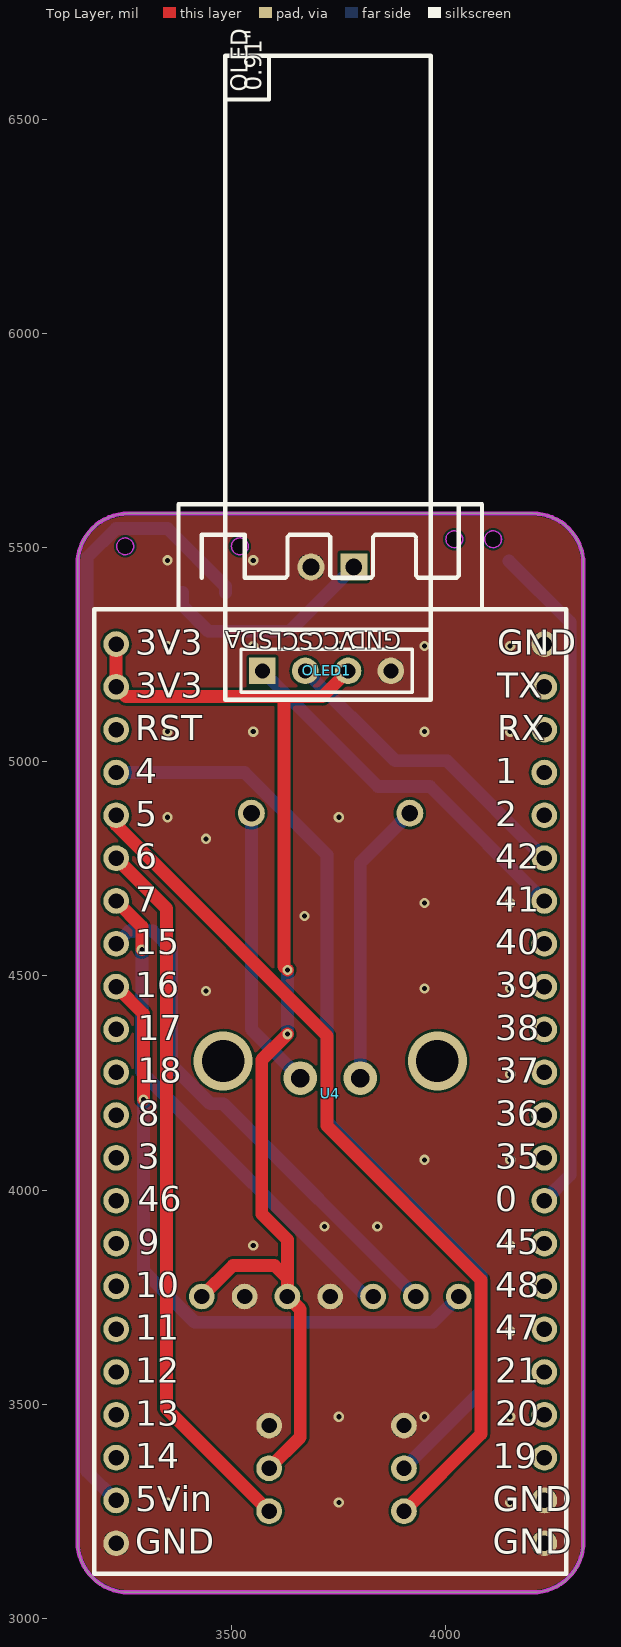
[diagram p0: Top Layer view]
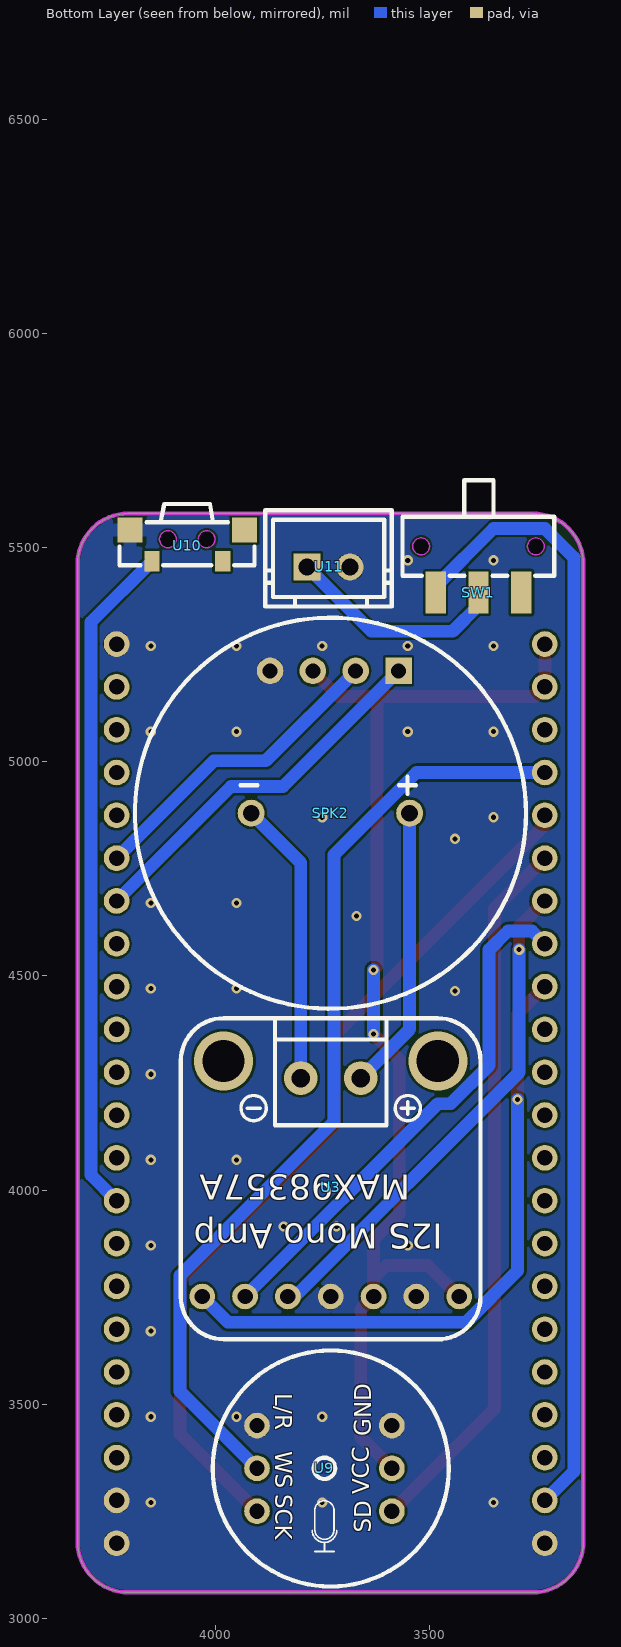
[diagram p1: Bottom Layer view, seen from below]
# Altium PCB MISC49945.pcbdoc
Units mil, origin at the board's own origin, x right, y up, seen from the top; angles counter-clockwise.
Board outline 1181.1 x 2519.68 mil, 2 copper layers (Top Layer, Bottom Layer), stack 62.206 mil thick; 8 components, 43 nets, 74 pads, 40 vias.

## Layer stack, top to bottom
Top Solder Mask Layer: solder mask 0.394, Dk 3.3
Top Layer: signal copper 1.379
Dielectric1: surface 59.449, FR4, Dk 4.5
Bottom Layer: signal copper 1.378
Bottom Solder Mask Layer: solder mask 0.394, Dk 3.3

## Board outline
3258.11,5580 ccw(c3258.11,5461.89) 3140,5461.89 3140,3178.43 ccw(c3258.11,3178.43) 3258.11,3060.32 4202.99,3060.32 ccw(c4202.99,3178.43) 4321.1,3178.43 4321.1,5461.89 ccw(c4202.99,5461.89) 4202.99,5580

## Design rules (kind name [scope] priority, off if disabled: settings)
BoardOutlineClearance Plane_Default_1 [All] p2 off: genericclearance=6 ignorepadtopadclearanceinfootprint=FALSE except(0: Arc-SplitContinuation Track-SplitContinuation SMDPad-SplitContinuation THPad-SplitContinuation Via-SplitContinuation Fill-SplitContinuation Region-SplitContinuation Poly-SplitContinuation Text-SplitContinuation Hole-SplitContinuation; 6: Arc-OutlineEdge Track-OutlineEdge SMDPad-OutlineEdge THPad-OutlineEdge Via-OutlineEdge Fill-OutlineEdge Region-OutlineEdge Poly-OutlineEdge Text-OutlineEdge Hole-OutlineEdge Arc-CutoutEdge Track-CutoutEdge SMDPad-CutoutEdge THPad-CutoutEdge Via-CutoutEdge Fill-CutoutEdge Region-CutoutEdge Poly-CutoutEdge Text-CutoutEdge Hole-CutoutEdge)
BoardOutlineClearance Copper_Default_1 [All] p4 off: genericclearance=6 ignorepadtopadclearanceinfootprint=FALSE except(0: Arc-SplitContinuation Track-SplitContinuation SMDPad-SplitContinuation THPad-SplitContinuation Via-SplitContinuation Fill-SplitContinuation Region-SplitContinuation Poly-SplitContinuation Text-SplitContinuation Hole-SplitContinuation; 6: Arc-OutlineEdge Track-OutlineEdge SMDPad-OutlineEdge THPad-OutlineEdge Via-OutlineEdge Fill-OutlineEdge Region-OutlineEdge Poly-OutlineEdge Text-OutlineEdge Hole-OutlineEdge Arc-CutoutEdge Track-CutoutEdge SMDPad-CutoutEdge THPad-CutoutEdge Via-CutoutEdge Fill-CutoutEdge Region-CutoutEdge Poly-CutoutEdge Text-CutoutEdge Hole-CutoutEdge)
BoardOutlineClearance Copper_gge24019_1 [All] p6 off: genericclearance=6 ignorepadtopadclearanceinfootprint=FALSE except(0: Arc-SplitContinuation Track-SplitContinuation SMDPad-SplitContinuation THPad-SplitContinuation Via-SplitContinuation Fill-SplitContinuation Region-SplitContinuation Poly-SplitContinuation Text-SplitContinuation Hole-SplitContinuation; 6: Arc-OutlineEdge Track-OutlineEdge SMDPad-OutlineEdge THPad-OutlineEdge Via-OutlineEdge Fill-OutlineEdge Region-OutlineEdge Text-OutlineEdge Hole-OutlineEdge Arc-CutoutEdge Track-CutoutEdge SMDPad-CutoutEdge THPad-CutoutEdge Via-CutoutEdge Fill-CutoutEdge Region-CutoutEdge Text-CutoutEdge Hole-CutoutEdge; 10: Poly-OutlineEdge Poly-CutoutEdge)
BoardOutlineClearance Default_1 [All] p8: genericclearance=6 ignorepadtopadclearanceinfootprint=FALSE except(0: Arc-SplitContinuation Track-SplitContinuation SMDPad-SplitContinuation THPad-SplitContinuation Via-SplitContinuation Fill-SplitContinuation Region-SplitContinuation Poly-SplitContinuation Text-SplitContinuation Hole-SplitContinuation; 6: Arc-OutlineEdge Track-OutlineEdge SMDPad-OutlineEdge THPad-OutlineEdge Via-OutlineEdge Fill-OutlineEdge Region-OutlineEdge Poly-OutlineEdge Text-OutlineEdge Hole-OutlineEdge Arc-CutoutEdge Track-CutoutEdge SMDPad-CutoutEdge THPad-CutoutEdge Via-CutoutEdge Fill-CutoutEdge Region-CutoutEdge Poly-CutoutEdge Text-CutoutEdge Hole-CutoutEdge)
Clearance Plane_Default [All] p1 off: gap=6 ignorepadtopadclearanceinfootprint=FALSE
Clearance Copper_Default [All] p3 off: gap=6 ignorepadtopadclearanceinfootprint=FALSE
Clearance Copper_gge24019 [All] p5 off: gap=6 ignorepadtopadclearanceinfootprint=FALSE except(10: Poly-Track Poly-SMDPad Poly-THPad Poly-Via Poly-Fill Poly-Region Poly-Poly Poly-Arc Poly-Text Poly-Hole)
Clearance Default [All] p7: gap=6 ignorepadtopadclearanceinfootprint=FALSE
DiffPairsRouting differentialPair [All] p1: maxlimit=6 minlimit=6 mostfreqgap=6 toplayer_minwidth=5 toplayer_prefwidth=10 toplayer_maxwidth=100 toplayer_mingap=6 toplayer_prefgap=6 toplayer_maxgap=6 bottomlayer_minwidth=5 bottomlayer_prefwidth=10 bottomlayer_maxwidth=100 bottomlayer_mingap=6 bottomlayer_prefgap=6 bottomlayer_maxgap=6 maxuncoupledlength=10
HoleToHoleClearance otherClearance [All] p1: gap=11.8 allowstackedmicrovias=TRUE
Length netLength [All] p1: minlimit=0 maxlimit=0
PasteMaskExpansion Common [All] p1: expansion=0
PlaneConnect Default_4 [All] p1: planeconnectstyle=Relief reliefexpansion=20 reliefentries=4 reliefconductorwidth=0 reliefairgap=10
PolygonConnect gge24019 [All] p1 off: connectstyle=Relief reliefconductorwidth=0 reliefentries=4 polygonreliefangle="90 Angle" airgapwidth=1 smdpad.connectstyle=Relief smdpad.reliefconductorwidth=0 smdpad.reliefentries=4 smdpad.polygonreliefangle="90 Angle" smdpad.airgapwidth=10 via.connectstyle=Relief via.reliefconductorwidth=10 via.reliefentries=4 via.polygonreliefangle="90 Angle" via.airgapwidth=10
PolygonConnect Default_5 [All] p2: connectstyle=Relief reliefconductorwidth=0 reliefentries=4 polygonreliefangle="90 Angle" airgapwidth=1 smdpad.connectstyle=Relief smdpad.reliefconductorwidth=0 smdpad.reliefentries=4 smdpad.polygonreliefangle="90 Angle" smdpad.airgapwidth=10 via.connectstyle=Relief via.reliefconductorwidth=10 via.reliefentries=4 via.polygonreliefangle="90 Angle" via.airgapwidth=10
RoutingVias Default_3 [All] p1: holewidth=12 width=24 viastyle="Through Hole" minholewidth=12 minwidth=24 maxholewidth=2362 maxwidth=3938
SolderMaskExpansion Common_1 [IsVia] p1: expansion=-1000 istentingtop=TRUE
SolderMaskExpansion Common_1 [All] p2: expansion=2 istentingtop=FALSE
Width Default_2 [All] p1: maxlimit=1000 minlimit=10 preferedwidth=30

## Components (designator, comment, footprint, x,y, rotation, side; value= is the part's Value field where it differs from the comment)
OLED1 "OLED0.91or0.96" OLED0.91 3485,5145 r90 top
SPK2 "FS-2308" BEEP-TH_BD23.2-P9.20-D1.0 3730.73,4880 r180 bottom
SW1 "SSSS211603" SW-SMD_SSSS211603 3385,5395 r180 bottom
U3 "Adafruit MAX98357 I2S Amp" "MAX98357 I2S AMP MODULE" 3730,3751.3 r90 bottom
U4 "NO" ESP32S3 3730,4230 r0 top
U9 "INMP441" INMP441 3744.7,3350 r180 bottom
U10 "GT-TC054A-H038-L1" SW-SMD_L7.8-W3.5-P4.20-EH 4065,5505 r180 bottom
U11 "_x001F_XH2.54-2P" CONN-TH_2P-P2.54-V 3735,5455 r180 bottom

## Footprints (in the part's own frame and the unit in brackets; to place one, negate y for a bottom-side part, rotate by r counter-clockwise, add the part's x,y. Pads: shape width x height; smd on the part's side, far side on the other; paste and mask are expansions set on the pad)
BEEP-TH_BD23.2-P9.20-D1.0 [mm]
  round 1.6 hole 1: 1(4.7,0) 2(-4.7,0)
  silkscreen extent -11.6,-11.6 11.6,11.6
CONN-TH_2P-P2.54-V [mm]
  rect 1.6x1.6 hole 1: 1(-1.27,0)
  round 1.6 hole 1: 2(1.27,0)
  silkscreen extent -3.75,-2.34 3.75,3.36
ESP32S3 [mil]
  round 60 hole 36: 1(-500,-1055) 2(-500,-955) 3(-500,-855) 4(-500,-755) 5(-500,-655) 6(-500,-555) 7(-500,-455) 8(-500,-355) 9(-500,-255) 10(-500,-155) 11(-500,-55) 12(-500,45) 13(-500,145) 14(-500,245) 15(-500,345) 16(-500,445) 17(-500,545) 18(-500,645) 19(-500,745) 20(-500,845) 21(-500,945) 22(-500,1045) 23(500,-1055) 24(500,-955) 25(500,-855) 26(500,-755) 27(500,-655) 28(500,-555) 29(500,-455) 30(500,-355) 31(500,-255) 32(500,-155) 33(500,-55) 34(500,45) 35(500,145) 36(500,245) 37(500,345) 38(500,445) 39(500,545) 40(500,645) 41(500,745) 42(500,845) 43(500,945) 44(500,1045)
  silkscreen extent -551,-1126 551,1371
INMP441 [mil]
  round 60 hole 36: 1(157.47,100) 2(157.47,0) 3(157.47,-100) 4(-157.49,100) 5(-157.49,0) 6(-157.49,-100)
  silkscreen extent -261,-276 290,275
"MAX98357 I2S AMP MODULE" [mil]
  round 60 hole 36: 1(0,300) 2(0,200) 3(0,100) 4(0,0) 5(0,-100) 6(0,-200) 7(0,-300)
  round 78.74 hole 43.31 paste+0 mask+4: 8(510,-70) 9(510,70)
  silkscreen extent -100,-350 650,350
OLED0.91 [mil]
  rect 62x62 hole 35 copper offset 0.04,-0.03 paste+0 mask+4: 1(67.32,-86.61)
  round 62 hole 35 copper offset 0.04,-0.03 paste+0 mask+4: 2(67.32,-186.61) 3(67.32,-286.61) 4(67.32,-386.61)
  silkscreen extent 0,-480 1504,0
SW-SMD_L7.8-W3.5-P4.20-EH [mm]
  rect 0.9x1.2 smd: 1(-2.1,-0.925) 2(2.1,-0.925)
  rect 1.5x1.5 smd: 3(-3.4,0.925) 4(3.4,0.925)
  Board Outline Layer circle w0.003: c1.15,0.375 r0.5
  Board Outline Layer circle w0.003: c-1.15,0.375 r0.5
  Board Outline Layer region: 0.65,0.375 0.7,0.158 0.838,-0.016 1.039,-0.112 1.261,-0.112 1.462,-0.016 1.601,0.158 1.65,0.375 1.65,0.375 1.601,0.592 1.462,0.766 1.261,0.862 1.039,0.862 0.838,0.766 0.7,0.592 0.65,0.375
  Board Outline Layer region: 0.65,0.375 0.66,0.277 0.688,0.184 0.734,0.097 0.797,0.021 0.872,-0.041 0.959,-0.087 1.053,-0.115 1.15,-0.125 1.248,-0.115 1.341,-0.087 1.428,-0.041 1.504,0.021 1.566,0.097 1.612,0.184 1.641,0.277 1.65,0.375 1.641,0.473 1.612,0.566 1.566,0.653 1.504,0.729 1.428,0.791 1.341,0.837 1.248,0.865 1.15,0.875 1.053,0.865 0.959,0.837 0.872,0.791 0.797,0.729 0.734,0.653 0.688,0.566 0.66,0.473
  Board Outline Layer region: -1.65,0.375 -1.601,0.158 -1.462,-0.016 -1.261,-0.112 -1.039,-0.112 -0.838,-0.016 -0.7,0.158 -0.65,0.375 -0.65,0.375 -0.7,0.592 -0.838,0.766 -1.039,0.862 -1.261,0.862 -1.462,0.766 -1.601,0.592 -1.65,0.375
  Board Outline Layer region: -1.65,0.375 -1.641,0.277 -1.612,0.184 -1.566,0.097 -1.504,0.021 -1.428,-0.041 -1.341,-0.087 -1.248,-0.115 -1.15,-0.125 -1.053,-0.115 -0.959,-0.087 -0.872,-0.041 -0.797,0.021 -0.734,0.097 -0.688,0.184 -0.66,0.277 -0.65,0.375 -0.66,0.473 -0.688,0.566 -0.734,0.653 -0.797,0.729 -0.872,0.791 -0.959,0.837 -1.053,0.865 -1.15,0.875 -1.248,0.865 -1.341,0.837 -1.428,0.791 -1.504,0.729 -1.566,0.653 -1.612,0.566 -1.641,0.473
  Multi-Layer board cut-out: 0.65,0.375 0.7,0.158 0.838,-0.016 1.039,-0.112 1.261,-0.112 1.462,-0.016 1.601,0.158 1.65,0.375 1.65,0.375 1.601,0.592 1.462,0.766 1.261,0.862 1.039,0.862 0.838,0.766 0.7,0.592 0.65,0.375
  Multi-Layer board cut-out: -1.65,0.375 -1.601,0.158 -1.462,-0.016 -1.261,-0.112 -1.039,-0.112 -0.838,-0.016 -0.7,0.158 -0.65,0.375 -0.65,0.375 -0.7,0.592 -0.838,0.766 -1.039,0.862 -1.261,0.862 -1.462,0.766 -1.601,0.592 -1.65,0.375
  silkscreen extent -4.02,-1.16 3.98,2.46
SW-SMD_SSSS211603 [mm]
  rect 1.2x2.5 smd: 1(-2.54,0) 2(0,0) 3(2.54,0)
  Board Outline Layer circle w0.003: c-3.401,2.75 r0.5
  Board Outline Layer circle w0.003: c3.401,2.75 r0.5
  Board Outline Layer region: -3.901,2.75 -3.852,2.533 -3.713,2.359 -3.512,2.263 -3.29,2.263 -3.089,2.359 -2.951,2.533 -2.901,2.75 -2.901,2.75 -2.951,2.967 -3.089,3.141 -3.29,3.238 -3.512,3.238 -3.713,3.141 -3.852,2.967 -3.901,2.75
  Board Outline Layer region: -3.901,2.75 -3.891,2.653 -3.863,2.559 -3.817,2.472 -3.755,2.397 -3.679,2.334 -3.592,2.288 -3.499,2.26 -3.401,2.25 -3.304,2.26 -3.21,2.288 -3.123,2.334 -3.048,2.397 -2.985,2.472 -2.939,2.559 -2.911,2.653 -2.901,2.75 -2.911,2.848 -2.939,2.941 -2.985,3.028 -3.048,3.104 -3.123,3.166 -3.21,3.212 -3.304,3.24 -3.401,3.25 -3.499,3.24 -3.592,3.212 -3.679,3.166 -3.755,3.104 -3.817,3.028 -3.863,2.941 -3.891,2.848
  Board Outline Layer region: 2.901,2.75 2.951,2.533 3.089,2.359 3.29,2.263 3.512,2.263 3.713,2.359 3.852,2.533 3.901,2.75 3.901,2.75 3.852,2.967 3.713,3.141 3.512,3.238 3.29,3.238 3.089,3.141 2.951,2.967 2.901,2.75
  Board Outline Layer region: 2.901,2.75 2.911,2.653 2.939,2.559 2.985,2.472 3.048,2.397 3.123,2.334 3.21,2.288 3.304,2.26 3.401,2.25 3.499,2.26 3.592,2.288 3.679,2.334 3.755,2.397 3.817,2.472 3.863,2.559 3.891,2.653 3.901,2.75 3.891,2.848 3.863,2.941 3.817,3.028 3.755,3.104 3.679,3.166 3.592,3.212 3.499,3.24 3.401,3.25 3.304,3.24 3.21,3.212 3.123,3.166 3.048,3.104 2.985,3.028 2.939,2.941 2.911,2.848
  Multi-Layer board cut-out: -3.901,2.75 -3.852,2.533 -3.713,2.359 -3.512,2.263 -3.29,2.263 -3.089,2.359 -2.951,2.533 -2.901,2.75 -2.901,2.75 -2.951,2.967 -3.089,3.141 -3.29,3.238 -3.512,3.238 -3.713,3.141 -3.852,2.967 -3.901,2.75
  Multi-Layer board cut-out: 2.901,2.75 2.951,2.533 3.089,2.359 3.29,2.263 3.512,2.263 3.713,2.359 3.852,2.533 3.901,2.75 3.901,2.75 3.852,2.967 3.713,3.141 3.512,3.238 3.29,3.238 3.089,3.141 2.951,2.967 2.901,2.75
  silkscreen extent -4.5,1 4.5,6.67

## Via types
v1: diameter 24, hole 12, Top Layer to Bottom Layer, 33 vias
v2: diameter 24.02, hole 12, Top Layer to Bottom Layer, 5 vias
v3: diameter 137.8, hole 98.4, Top Layer to Bottom Layer, 2 vias

## Nets (pads, with @x,y where several pads share a name; then routed paths per layer and width w, separated by ;. In a path a pad name is that pad's centre, name@x,y a point inside that pad or via, vN(x,y) a via of type N, cw(c..) or ccw(c..) an arc to the next point about the centre after c; other vN are vias at no path point)
0: U4.31 U10.1 | length 1577.4
  Bottom Layer w30: U10.1 4290,5326.27 4290,4035 U4.31
1: U4.41
2: U4.40
3: U4.10
3.3V: OLED1.3 U3.5 U3.7 U4.21 U4.22 U9.2 | length 2816.5
  Top Layer w30: U4.22 U4.21 3252.64,5152.36 3621.64,5152.36 ; U3.7 3502.7,3824 3600,3824 3630,3794 ; U9.2 3660,3422.78 3660,3721.3 U3.5 3630,3794 ; v1(3630,4364) 3570,4304 3570,3944 3630,3884 3630,3794 ; v1(3630,4514) 3621.64,4522.36 3621.64,5152.36 ; OLED1.3@3771.64,5212.36 3711.64,5152.36 3621.64,5152.36
  Bottom Layer w30: v1(3630,4364) v1(3630,4514)
4: U4.19 U9.5 | length 2228.3
  Bottom Layer w30: U4.19 3530,4975 3722.18,4782.82 3722.18,4160 4082.18,3800 4082.18,3530 U9.5
5: U4.18 U9.6 | length 2052.5
  Top Layer w30: U4.18 3230,4852.18 3722.18,4360 3722.18,4150 4082.18,3790 4082.18,3430 U9.6
5V-VIN: SW1.1 U4.2 | length 2652.1
  Bottom Layer w30: U4.2 3162.22,3342.78 3162.22,5477.22 3230,5545 3350,5545 3485,5410 SW1.1
6: U4.17 U9.3 | length 1673
  Top Layer w30: U4.17 3347.22,4657.78 3347.22,3490 U9.3
7: U3.3 U4.16 | length 1181.8
  Top Layer w30: U4.16 3290,4615 v1(3290,4561.31)
  Bottom Layer w30: v1(3290,4561.31) 3290,4275 3813.7,3751.3 U3.3
8: U4.11
9: U4.8
10: U4.7
11: U4.6
12: U4.5
13: U4.4
14: U4.3
15: U3.2 U4.15 | length 1224.2
  Bottom Layer w30: U4.15 3260,4605 3316.3,4605 3360,4561.31 3360,4291.31 3450,4201.31 3480,4201.31 U3.2
16: U3.1 U4.14 | length 1500.9
  Top Layer w30: U4.14 3293.7,4411.31 v1(3293.7,4211.31)
  Bottom Layer w30: v1(3293.7,4211.31) 3293.7,3811.3 3413.7,3691.3 3970,3691.3 U3.1
17: U4.13
18: U4.12
19: U4.25
20: U4.26
21: U4.27
35: U4.32
36: U4.33
37: U4.34
38: U4.35
39: U4.36
40: U4.37
41: OLED1.1 U4.38 | length 880.9
  Bottom Layer w30: OLED1.1@3571.64,5212.36 3841.64,4942.36 3962.64,4942.36 U4.38
42: OLED1.2 U4.39 | length 739.5
  Bottom Layer w30: OLED1.2@3671.64,5212.36 3881.64,5002.36 4002.64,5002.36 U4.39
45: U4.30
46: U4.9
47: U4.28
48: U4.29
$1N2378: SW1.2 U11.1 | length 517
  Bottom Layer w30: SW1.2 3385,5365 3445,5305 3635,5305 U11.1
GND: OLED1.4 U3.4 U3.6 U4.1 U4.23 U4.24 U4.44 U9.1 U9.4 U10.3 U11.2
  other v1: 3350.1,3270.41 3750.1,3270.41 4150.1,3270.41 3750.1,3470.41 3950.1,3470.41 4150.1,3470.41 4150.1,3670.41 3550.1,3870.41 4150.1,3870.41 3950.1,4070.41 4150.1,4070.41 4150.1,4270.41 3950.1,4470.41 4150.1,4470.41 3950.1,4670.41 4150.1,4670.41 3350.1,4870.41 3750.1,4870.41 3350.1,5070.41 3550.1,5070.41 3950.1,5070.41 4150.1,5070.41 3350.1,5270.41 3550.1,5270.41 3750.1,5270.41 3950.1,5270.41 4150.1,5270.41 3350.1,5470.41 3550.1,5470.41
  other v2: 3716.38,3915 3840,3915 3440,4464.68 3670,4640 3440,4820
RST: U4.20
RX: U4.42
SPEAKER+: SPK2.1 U3.8 | length 666
  Bottom Layer w30: SPK2.1 3545.69,4375.61 U3.8
SPEAKER-: SPK2.2 U3.9 | length 666.6
  Bottom Layer w30: U3.9 3800,4764.23 SPK2.2
TX: U4.43
pads on no net: SW1.3 U10.2 U10.4
copper on no net:
  other v3: 3480,4301.31 3980,4301.31

## Polygon pours and split planes (outlines as drawn)
GND on Bottom Layer (solid, remove dead copper, pour order 2): 3000,5705 3000,3020 4505,3020 4505,5705
GND on Top Layer (solid, remove dead copper, pour order 0): 3030,5630 3030,3000 4465,3000 4465,5630

## Keep-outs
Board Outline Layer:
  the board outline again, w10